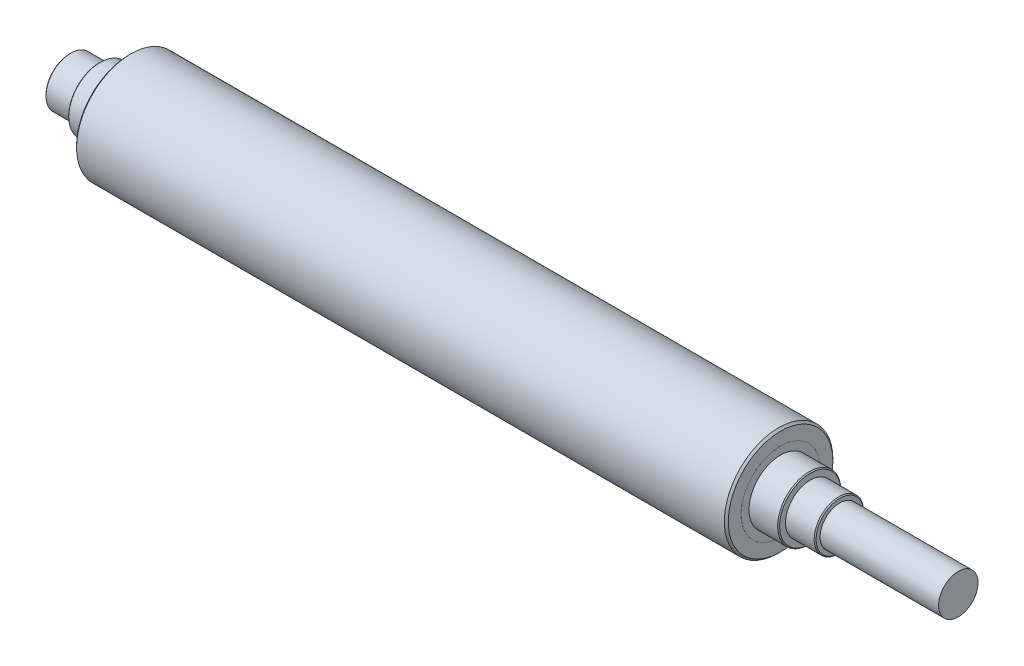
from build123d import *

# Parameters (mm, degrees)
SKETCH2_R           = 27.5
SKETCH2_R_2         = 20
BOSS_EXTRUDE1_DEPTH = 330
CHAMFER1_SIZE       = 0.5
CHAMFER2_SIZE       = 1


with BuildPart() as part:
    # Sketch1 → Revolve1 (revolve)
    with BuildSketch(Plane.XY, mode=Mode.PRIVATE) as revolve1_sk:
        Polygon((450, 10), (390, 10), (390, 12.5), (375, 12.5), (375, 16), (360, 16), (360, 20), (30, 20), (30, 16), (15, 16), (15, 12.5), (0, 12.5), (0, 0), (450, 0), align=None)
    revolve(revolve1_sk.sketch.rotate(Axis((0, 0, 0), (1, 0, 0)), 90), axis=Axis((0, 0, 0), (1, 0, 0)))

    # Chamfer1
    chamfer1_edges = [part.edges().sort_by_distance(p)[0] for p in [
        (15, 0, -16),
        (375, 0, -16),
        (390, 0, -12.5),
        (0, 0, -12.5),
    ]]
    chamfer(chamfer1_edges, length=CHAMFER1_SIZE)


with BuildPart() as body_2:
    # Sketch2 → Boss-Extrude1 (new body)
    with BuildSketch(Plane(origin=(360, 0, 0), x_dir=(0, 0, -1), z_dir=(1, 0, 0))):
        Circle(SKETCH2_R)
        Circle(SKETCH2_R_2, mode=Mode.SUBTRACT)
    extrude(amount=-BOSS_EXTRUDE1_DEPTH)

    # Chamfer2
    chamfer2_edges = [body_2.edges().sort_by_distance(p)[0] for p in [
        (360, 0, 27.5),
        (30, 0, 27.5),
    ]]
    chamfer(chamfer2_edges, length=CHAMFER2_SIZE)


solid = Compound([part.part, body_2.part])
